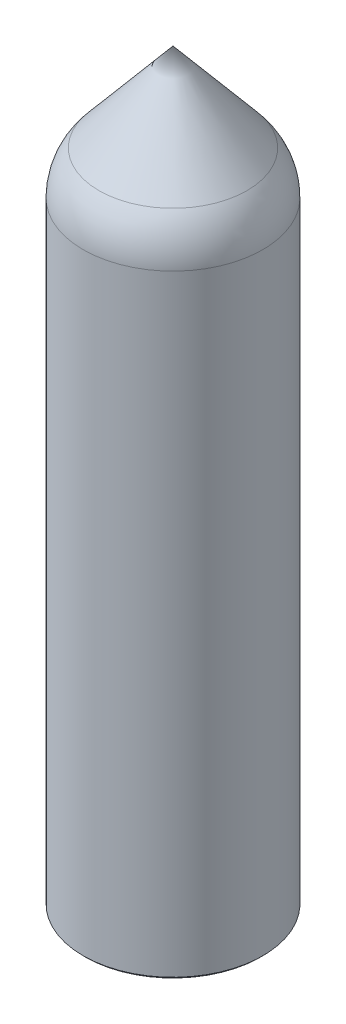
SolidWorks part; units mm, degrees
ref_plane "Front Plane" through (0, 0, 0) normal (0, 0, 1) x (1, 0, 0)
ref_plane "Top Plane" through (0, 0, 0) normal (0, 1, 0) x (1, 0, 0)
ref_plane "Right Plane" through (0, 0, 0) normal (1, 0, 0) x (0, 0, -1)
sketch "Sketch1" plane through (0, 0, 0) normal (0, 0, 1) x (1, 0, 0)
  line L0 (0, 0) -> (-20, -23.8351)
  line L1 (-20, -23.8351) -> (-20, -166)
  line L2 (-20, -166) -> (0, -166)
  line L3 (0, -166) -> (0, 0)
  dimension "D1" = 40
  dimension "D2" = 166
  dimension "D3" = 20
revolve "Revolve1" add sketch "Sketch1" angle 360 about L3
fillet "Fillet1" radius 15 1 edges at (0, -23.8351, -20)
chamfer "Chamfer1" distance 0.5 angle 45 1 edges at (0, -166, -20)
